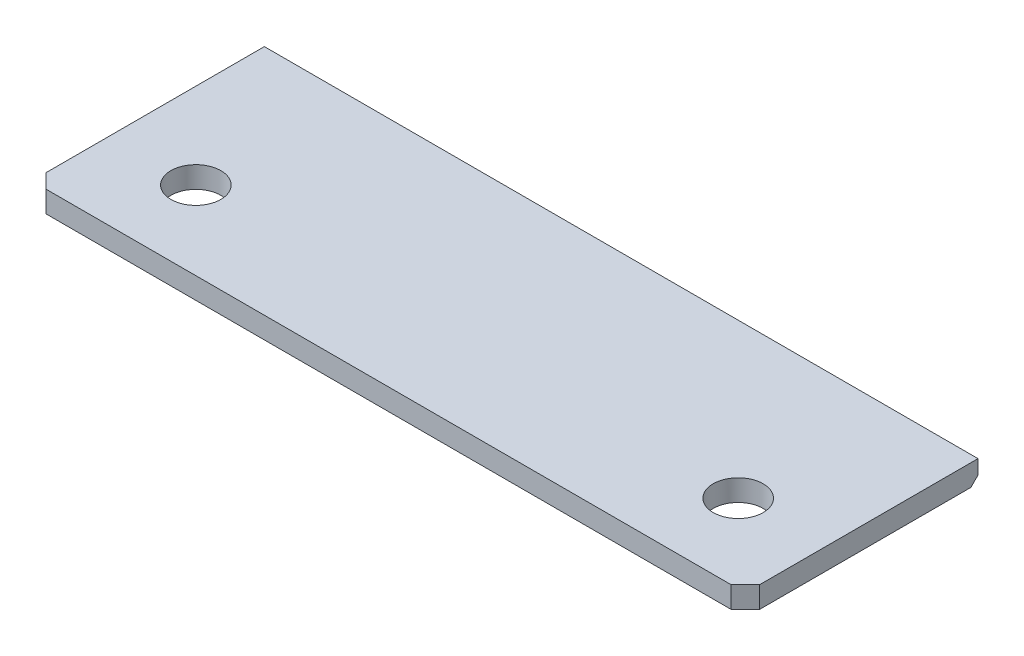
from build123d import *

# Parameters (mm, degrees)
SKETCH1_W           = 50
SKETCH1_H           = 16.3
BOSS_EXTRUDE1_DEPTH = 1.5
SKETCH3_R           = 1.75
CUT_EXTRUDE2_DEPTH  = 10
CHAMFER1_SIZE       = 1
CHAMFER2_SIZE       = 0.5


with BuildPart() as part:
    # Sketch1 → Boss-Extrude1 (new body)
    with BuildSketch(Plane(origin=(0, 0, 0), x_dir=(1, 0, 0), z_dir=(0, 1, 0))):
        Rectangle(SKETCH1_W, SKETCH1_H)
    extrude(amount=BOSS_EXTRUDE1_DEPTH)

    # Sketch3 → Cut-Extrude2 (cut)
    with BuildSketch(Plane(origin=(0, 1.5, 0), x_dir=(1, 0, 0), z_dir=(0, 1, 0))):
        with Locations(Location((-19, -2.65, 0), (0, 0, 270))):
            Circle(SKETCH3_R)
        with Locations(Location((19, -2.65, 0), (0, 0, 270))):
            Circle(SKETCH3_R)
    extrude(amount=-CUT_EXTRUDE2_DEPTH, mode=Mode.SUBTRACT)

    # Chamfer1
    chamfer1_edges = [part.edges().sort_by_distance(p)[0] for p in [
        (25, 0.75, 8.15),
        (-25, 0.75, 8.15),
    ]]
    chamfer(chamfer1_edges, length=CHAMFER1_SIZE)

    # Chamfer2
    chamfer2_edges = [part.edges().sort_by_distance(p)[0] for p in [
        (0, 0, -8.15),
    ]]
    chamfer(chamfer2_edges, length=CHAMFER2_SIZE)


solid = part.part
